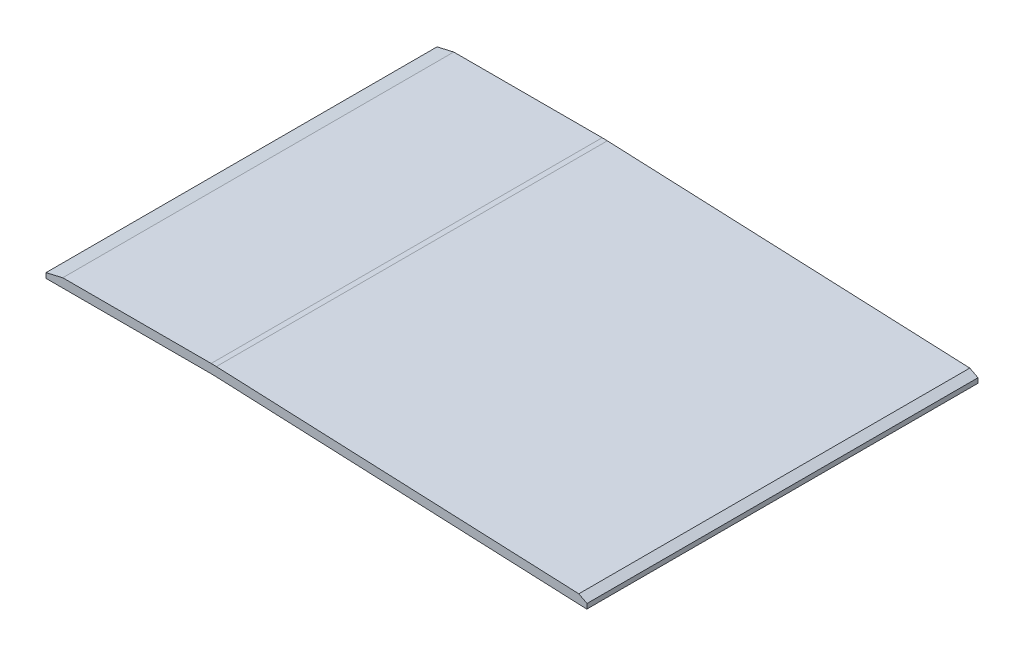
SolidWorks part; units mm, degrees
material "普通碳钢"
ref_plane "Front Plane" through (0, 0, 0) normal (0, 0, 1) x (1, 0, 0)
ref_plane "Top Plane" through (0, 0, 0) normal (0, 1, 0) x (1, 0, 0)
ref_plane "Right Plane" through (0, 0, 0) normal (1, 0, 0) x (0, 0, -1)
sketch "Sketch1" plane through (0, 0, 0) normal (0, 0, 1) x (1, 0, 0)
  line L0 (0, 0) -> (295.7069, 0)
  line L1 (304.9758, 15.801) -> (953.9004, -12.0711)
  line L2 (304.2892, -0.1842) -> (968.2, -28.7)
  line L3 (0, 0) -> (0, 9)
  line L4 (0, 9) -> (30, 16)
  line L5 (30, 16) -> (295.7069, 16)
  line L6 (968.2, -28.7) -> (968.5862, -19.7083)
  line L7 (953.9004, -12.0711) -> (968.5862, -19.7083)
  line L8 (0, -55) -> (0, 55) construction
  line L10 (304.9758, 15.801) -> (968.8866, -12.7147) construction
  arc A0 (304.2892, -0.1842) -> (295.7069, 0) centre (295.7069, -200) ccw
  arc A1 (304.9758, 15.801) -> (295.7069, 16) centre (295.7069, -200) ccw
  point P4 (306.2556, 15.7461)
  point P9 (968.8866, -12.7147)
  point P12 (497.7056, -4000)
  point P15 (817.474, 3.2492)
  point P21 (300, 0)
  dimension "D3" = 16
  dimension "D1" = 300
  dimension "D8" = 200
  dimension "D2" = 9
  dimension "D4" = 30
  dimension "D5" = 9
  dimension "D7" = 28.7
  dimension "D9" = 968.2
  dimension "D6" = 15
extrude "Boss-Extrude1" add sketch "Sketch1" along normal blind 700
sketch "Sketch2" plane through (0, 0, 0) normal (0, 1, 0) x (1, 0, 0)
  line L0 (65, 0) -> (65, -18)
  line L1 (-24.585, 0) -> (24.585, 0) construction
  line L2 (75, -28) -> (147, -28)
  line L3 (152, -33) -> (152, -79)
  line L4 (147, -84) -> (75, -84)
  line L5 (65, -94) -> (65, -120)
  line L6 (60, -125) -> (10, -125)
  line L7 (0, -700) -> (0, 0) construction
  line L8 (0, -135) -> (0, -565)
  line L9 (0, -350) -> (414.8964, -350) construction
  line L10 (60, -575) -> (10, -575)
  line L11 (65, -606) -> (65, -580)
  line L12 (147, -616) -> (75, -616)
  line L13 (152, -667) -> (152, -621)
  line L14 (75, -672) -> (147, -672)
  line L15 (65, -700) -> (65, -682)
  line L16 (65, 0) -> (-175.2836, 0)
  line L17 (-175.2836, 0) -> (-175.2836, -700)
  line L18 (-175.2836, -700) -> (65, -700)
  arc A0 (75, -84) -> (65, -94) centre (75, -94) ccw
  arc A1 (75, -28) -> (65, -18) centre (75, -18) cw
  arc A2 (60, -125) -> (65, -120) centre (60, -120) ccw
  arc A3 (147, -84) -> (152, -79) centre (147, -79) ccw
  arc A4 (152, -33) -> (147, -28) centre (147, -33) ccw
  arc A5 (10, -125) -> (0, -135) centre (10, -135) ccw
  arc A6 (10, -575) -> (0, -565) centre (10, -565) cw
  arc A7 (152, -667) -> (147, -672) centre (147, -667) cw
  arc A8 (147, -616) -> (152, -621) centre (147, -621) cw
  arc A9 (60, -575) -> (65, -580) centre (60, -580) cw
  arc A10 (75, -672) -> (65, -682) centre (75, -682) ccw
  arc A11 (75, -616) -> (65, -606) centre (75, -606) cw
  point P15 (65, -84)
  point P26 (0, -125)
  dimension "D3" = 10
  dimension "D4" = 5
  dimension "D5" = 10
  dimension "D1" = 152
  dimension "D2" = 65
  dimension "D6" = 450
  dimension "D7" = 532
  dimension "D8" = 644
  dimension "D9" = 240.2836
extrude "Cut-Extrude1" [suppressed] cut sketch "Sketch2" along normal through all
